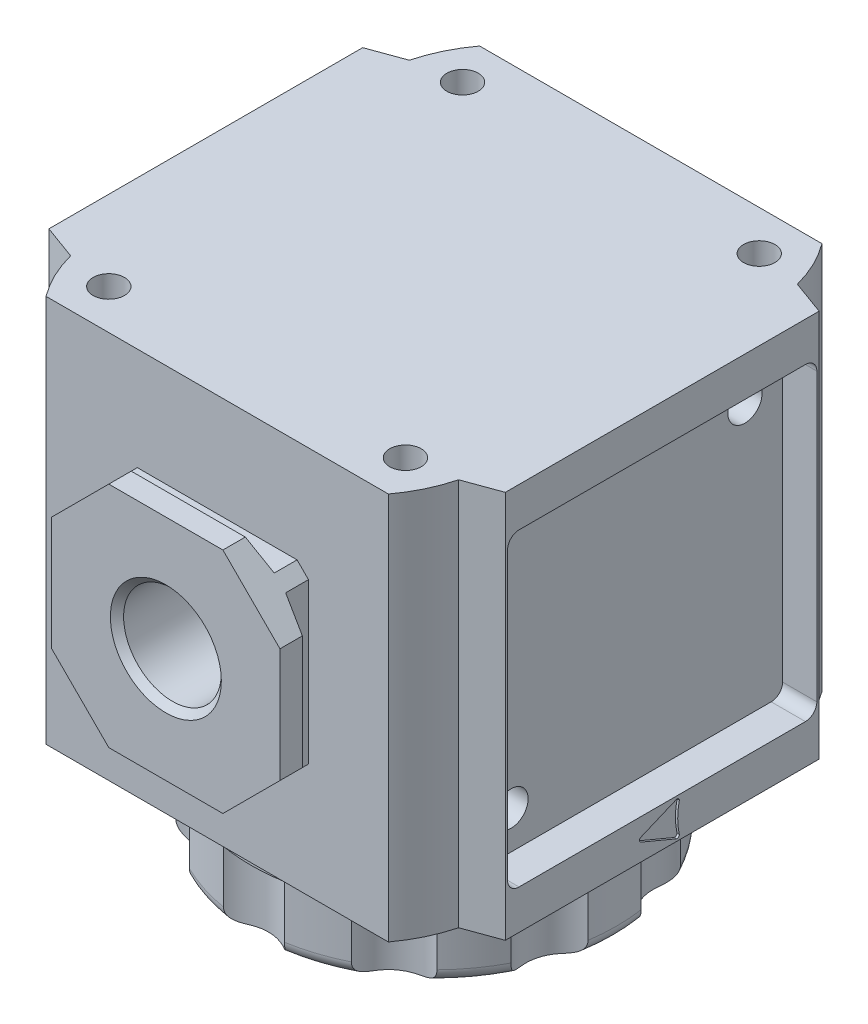
from build123d import *

# Parameters (mm, degrees)
EXTRUDE_1_DEPTH             = 17
EXTRUDE_1_DEPTH_BACK        = 17
EXTRUDE_2_DEPTH             = 17
EXTRUDE_2_DEPTH_BACK        = 17
EXTRUDE_3_DEPTH             = 17
EXTRUDE_3_DEPTH_BACK        = 17
SKETCH_5_R                  = 21.1
CUT_EXTRUDE_1_DEPTH         = 5.8
EXTRUDE_4_DEPTH             = 2
EXTRUDE_5_DEPTH             = 2.5
EXTRUDE_6_DEPTH             = 2
EXTRUDE_7_DEPTH             = 2.5
CUT_EXTRUDE_2_DEPTH         = 10
CUT_EXTRUDE_2_DEPTH_BACK    = 10
CUT_EXTRUDE_3_DEPTH         = 10
CUT_EXTRUDE_3_DEPTH_BACK    = 10
CUT_EXTRUDE_4_DEPTH         = 10
CUT_EXTRUDE_4_DEPTH_BACK    = 10
CUT_EXTRUDE_5_DEPTH         = 10
CUT_EXTRUDE_5_DEPTH_BACK    = 10
CUT_EXTRUDE_6_DEPTH         = 10
CUT_EXTRUDE_6_DEPTH_BACK    = 10
CUT_EXTRUDE_7_DEPTH         = 10
CUT_EXTRUDE_7_DEPTH_BACK    = 10
CUT_EXTRUDE_8_DEPTH         = 10
CUT_EXTRUDE_8_DEPTH_BACK    = 10
CUT_EXTRUDE_9_DEPTH         = 10
CUT_EXTRUDE_9_DEPTH_BACK    = 10
SKETCH_20_R                 = 1.5
CUT_EXTRUDE_10_DEPTH        = 6
SKETCH_21_R                 = 1.5
CUT_EXTRUDE_11_DEPTH        = 6
SKETCH_22_R                 = 1.375
CUT_EXTRUDE_12_DEPTH        = 3
PATTERN_LINEAR_1_COUNT      = 2
PATTERN_LINEAR_1_PITCH      = 26
PATTERN_LINEAR_1_COUNT_DIR2 = 2
PATTERN_LINEAR_1_PITCH_DIR2 = 31
SKETCH_24_R                 = 13
CUT_EXTRUDE_13_DEPTH        = 0.2
CUT_EXTRUDE_14_DEPTH        = 0.2
CUT_EXTRUDE_15_DEPTH        = 0.2
CUT_EXTRUDE_16_DEPTH        = 1
EXTRUDE_8_DEPTH             = 1
SKETCH_29_R                 = 1.5
CUT_EXTRUDE_17_DEPTH        = 0.5
SKETCH_31_R                 = 1.5
CUT_EXTRUDE_18_DEPTH        = 0.5
SKETCH_30_R                 = 0.271317829
CUT_EXTRUDE_19_DEPTH        = 0.2
CUT_EXTRUDE_20_DEPTH        = 3


with BuildPart() as part:
    # 草图1 → 凸台-拉伸1 (new, two sides: drawn at the far end of the back side and taken through both)
    with BuildSketch(Plane(origin=(0, 0, 0), x_dir=(1, 0, 0), z_dir=(0, 1, 0)).offset(-EXTRUDE_1_DEPTH_BACK)):
        with BuildLine():
            Line((-17, 14.841910703), (-17, -14.841910703))
            ThreePointArc((-17, -14.841910703), (-16.201733132, -17.017987001), (-15, -19))
            Line((-15, -19), (15, -19))
            ThreePointArc((15, -19), (16.201733132, -17.017987001), (17, -14.841910703))
            Line((17, -14.841910703), (17, 14.841910703))
            ThreePointArc((17, 14.841910703), (16.201733132, 17.017987001), (15, 19))
            Line((15, 19), (-15, 19))
            ThreePointArc((-15, 19), (-16.201733132, 17.017987001), (-17, 14.841910703))
        make_face()
    extrude(amount=EXTRUDE_1_DEPTH + EXTRUDE_1_DEPTH_BACK)

    # 草图2 → 凸台-拉伸2 (add, two sides: drawn at the far end of the back side and taken through both)
    with BuildSketch(Plane(origin=(0, 0, 0), x_dir=(1, 0, 0), z_dir=(0, 1, 0)).offset(-EXTRUDE_2_DEPTH_BACK)):
        Polygon((-20, -13.75), (-17, -14.841910703), (-17, 14.841910703), (-20, 13.75), align=None)
    extrude(amount=EXTRUDE_2_DEPTH + EXTRUDE_2_DEPTH_BACK)

    # 草图3 → 凸台-拉伸3 (add, two sides: drawn at the far end of the back side and taken through both)
    with BuildSketch(Plane(origin=(0, 0, 0), x_dir=(1, 0, 0), z_dir=(0, 1, 0)).offset(-EXTRUDE_3_DEPTH_BACK)):
        Polygon((17, 14.841910703), (17, -14.841910703), (20, -13.75), (20, 13.75), align=None)
    extrude(amount=EXTRUDE_3_DEPTH + EXTRUDE_3_DEPTH_BACK)

    # 草图4 → 旋转1 (revolve)
    with BuildSketch(Plane.XY, mode=Mode.PRIVATE) as revolve_1_sk:
        with BuildLine():
            Line((0, -17), (16.1, -17))
            Line((16.1, -17), (16.1, -19))
            Line((16.1, -19), (16, -19))
            Line((16, -19), (16, -24.8))
            ThreePointArc((16, -24.8), (15.648528137, -25.648528137), (14.8, -26))
            Line((14.8, -26), (0, -26))
            Line((0, -26), (0, -17))
        make_face()
    revolve(revolve_1_sk.sketch.rotate(Axis((0, -26, 0), (0, 1, 0)), 270), axis=Axis((0, -26, 0), (0, 1, 0)))

    # 草图5 → 切除-拉伸1 (cut)
    with BuildSketch(Plane(origin=(0, -26, 0), x_dir=(-1, 0, 0), z_dir=(0, -1, 0))):
        Circle(SKETCH_5_R)
        with BuildLine():
            ThreePointArc((15.830577633, -2.322242841), (16, 0), (15.830577633, 2.322242841))
            ThreePointArc((15.830577633, 2.322242841), (13.790319486, 4.480746418), (14.17218643, 7.426246145))
            ThreePointArc((14.17218643, 7.426246145), (12.94427191, 9.404564037), (11.442226242, 11.183713991))
            ThreePointArc((11.442226242, 11.183713991), (8.522886158, 11.730746418), (7.100501705, 14.338161512))
            ThreePointArc((7.100501705, 14.338161512), (4.94427191, 15.216904261), (2.683333333, 15.773386517))
            ThreePointArc((2.683333333, 15.773386517), (0, 14.5), (-2.683333333, 15.773386517))
            ThreePointArc((-2.683333333, 15.773386517), (-4.94427191, 15.216904261), (-7.100501705, 14.338161512))
            ThreePointArc((-7.100501705, 14.338161512), (-8.522886158, 11.730746418), (-11.442226242, 11.183713991))
            ThreePointArc((-11.442226242, 11.183713991), (-12.94427191, 9.404564037), (-14.17218643, 7.426246145))
            ThreePointArc((-14.17218643, 7.426246145), (-13.790319486, 4.480746418), (-15.830577633, 2.322242841))
            ThreePointArc((-15.830577633, 2.322242841), (-16, 0), (-15.830577633, -2.322242841))
            ThreePointArc((-15.830577633, -2.322242841), (-13.790319486, -4.480746418), (-14.17218643, -7.426246145))
            ThreePointArc((-14.17218643, -7.426246145), (-12.94427191, -9.404564037), (-11.442226242, -11.183713991))
            ThreePointArc((-11.442226242, -11.183713991), (-8.522886158, -11.730746418), (-7.100501705, -14.338161512))
            ThreePointArc((-7.100501705, -14.338161512), (-4.94427191, -15.216904261), (-2.683333333, -15.773386517))
            ThreePointArc((-2.683333333, -15.773386517), (0, -14.5), (2.683333333, -15.773386517))
            ThreePointArc((2.683333333, -15.773386517), (4.94427191, -15.216904261), (7.100501705, -14.338161512))
            ThreePointArc((7.100501705, -14.338161512), (8.522886158, -11.730746418), (11.442226242, -11.183713991))
            ThreePointArc((11.442226242, -11.183713991), (12.94427191, -9.404564037), (14.17218643, -7.426246145))
            ThreePointArc((14.17218643, -7.426246145), (13.790319486, -4.480746418), (15.830577633, -2.322242841))
        make_face(mode=Mode.SUBTRACT)
    extrude(amount=-CUT_EXTRUDE_1_DEPTH, mode=Mode.SUBTRACT)

    # 草图6 → 凸台-拉伸4 (add)
    with BuildSketch(Plane.XY.offset(19)):
        Polygon((-8, -7), (-7, -8), (7, -8), (8, -7), (8, 7), (7, 8), (-7, 8), (-8, 7), align=None)
    extrude(amount=EXTRUDE_4_DEPTH)

    # 草图7 → 凸台-拉伸5 (add)
    with BuildSketch(Plane.XY.offset(21)):
        Polygon((-10, -5), (-5, -10), (5, -10), (10, -5), (10, 5), (5, 10), (-5, 10), (-10, 5), align=None)
    extrude(amount=EXTRUDE_5_DEPTH)

    # 草图8 → 凸台-拉伸6 (add)
    with BuildSketch(Plane.XY.offset(-19)):
        Polygon((-8, -7), (-7, -8), (7, -8), (8, -7), (8, 7), (7, 8), (-7, 8), (-8, 7), align=None)
    extrude(amount=-EXTRUDE_6_DEPTH)

    # 草图9 → 凸台-拉伸7 (add)
    with BuildSketch(Plane.XY.offset(-21)):
        Polygon((-10, -5), (-5, -10), (5, -10), (10, -5), (10, 5), (5, 10), (-5, 10), (-10, 5), align=None)
    extrude(amount=-EXTRUDE_7_DEPTH)

    # 草图10 → 切除-拉伸2 (cut, two sides: drawn at the far end of the back side and taken through both)
    with BuildSketch(Plane(origin=(0, 0, 0), x_dir=(0, 0, -1), z_dir=(1, 0, 0)).offset(-CUT_EXTRUDE_2_DEPTH_BACK)):
        Polygon((-21.535898385, 10), (-21, 8), (-21, 10), align=None)
    extrude(amount=CUT_EXTRUDE_2_DEPTH + CUT_EXTRUDE_2_DEPTH_BACK, mode=Mode.SUBTRACT)

    # 草图11 → 切除-拉伸3 (cut, two sides: drawn at the far end of the back side and taken through both)
    with BuildSketch(Plane(origin=(0, 0, 0), x_dir=(0, 0, -1), z_dir=(1, 0, 0)).offset(-CUT_EXTRUDE_3_DEPTH_BACK)):
        Polygon((-21.535898385, -10), (-21, -10), (-21, -8), align=None)
    extrude(amount=CUT_EXTRUDE_3_DEPTH + CUT_EXTRUDE_3_DEPTH_BACK, mode=Mode.SUBTRACT)

    # 草图12 → 切除-拉伸4 (cut, two sides: drawn at the far end of the back side and taken through both)
    with BuildSketch(Plane(origin=(0, 0, 0), x_dir=(0, 0, -1), z_dir=(1, 0, 0)).offset(-CUT_EXTRUDE_4_DEPTH_BACK)):
        Polygon((21, 8), (21.535898385, 10), (21, 10), align=None)
    extrude(amount=CUT_EXTRUDE_4_DEPTH + CUT_EXTRUDE_4_DEPTH_BACK, mode=Mode.SUBTRACT)

    # 草图13 → 切除-拉伸5 (cut, two sides: drawn at the far end of the back side and taken through both)
    with BuildSketch(Plane(origin=(0, 0, 0), x_dir=(0, 0, -1), z_dir=(1, 0, 0)).offset(-CUT_EXTRUDE_5_DEPTH_BACK)):
        Polygon((21, -8), (21, -10), (21.535898385, -10), align=None)
    extrude(amount=CUT_EXTRUDE_5_DEPTH + CUT_EXTRUDE_5_DEPTH_BACK, mode=Mode.SUBTRACT)

    # 草图14 → 切除-拉伸6 (cut, two sides: drawn at the far end of the back side and taken through both)
    with BuildSketch(Plane(origin=(0, 0, 0), x_dir=(1, 0, 0), z_dir=(0, 1, 0)).offset(-CUT_EXTRUDE_6_DEPTH_BACK)):
        Polygon((8, 21), (10, 21), (10, 21.535898385), align=None)
    extrude(amount=CUT_EXTRUDE_6_DEPTH + CUT_EXTRUDE_6_DEPTH_BACK, mode=Mode.SUBTRACT)

    # 草图15 → 切除-拉伸7 (cut, two sides: drawn at the far end of the back side and taken through both)
    with BuildSketch(Plane(origin=(0, 0, 0), x_dir=(1, 0, 0), z_dir=(0, 1, 0)).offset(-CUT_EXTRUDE_7_DEPTH_BACK)):
        Polygon((-10, 21), (-8, 21), (-10, 21.535898385), align=None)
    extrude(amount=CUT_EXTRUDE_7_DEPTH + CUT_EXTRUDE_7_DEPTH_BACK, mode=Mode.SUBTRACT)

    # 草图16 → 切除-拉伸8 (cut, two sides: drawn at the far end of the back side and taken through both)
    with BuildSketch(Plane(origin=(0, 0, 0), x_dir=(1, 0, 0), z_dir=(0, 1, 0)).offset(-CUT_EXTRUDE_8_DEPTH_BACK)):
        Polygon((8, -21), (10, -21.535898385), (10, -21), align=None)
    extrude(amount=CUT_EXTRUDE_8_DEPTH + CUT_EXTRUDE_8_DEPTH_BACK, mode=Mode.SUBTRACT)

    # 草图17 → 切除-拉伸9 (cut, two sides: drawn at the far end of the back side and taken through both)
    with BuildSketch(Plane(origin=(0, 0, 0), x_dir=(1, 0, 0), z_dir=(0, 1, 0)).offset(-CUT_EXTRUDE_9_DEPTH_BACK)):
        Polygon((-10, -21), (-10, -21.535898385), (-8, -21), align=None)
    extrude(amount=CUT_EXTRUDE_9_DEPTH + CUT_EXTRUDE_9_DEPTH_BACK, mode=Mode.SUBTRACT)

    # 草图18 → 切除-旋转1 (revolve, cut)
    with BuildSketch(Plane(origin=(0, 0, 0), x_dir=(0, 0, -1), z_dir=(1, 0, 0)), mode=Mode.PRIVATE) as cut_revolve_1_sk:
        Polygon((14.5, 0), (14.5, 4.283), (22.919, 4.283), (23.5, 4.864), (23.5, 0), align=None)
    revolve(cut_revolve_1_sk.sketch.rotate(Axis((0, 0, -23.5), (0, 0, 1)), 270), axis=Axis((0, 0, -23.5), (0, 0, 1)), mode=Mode.SUBTRACT)

    # 草图19 → 切除-旋转2 (revolve, cut)
    with BuildSketch(Plane(origin=(0, 0, 0), x_dir=(0, 0, -1), z_dir=(1, 0, 0)), mode=Mode.PRIVATE) as cut_revolve_2_sk:
        Polygon((-23.5, 0), (-23.5, 4.864), (-22.919, 4.283), (-14.5, 4.283), (-14.5, 0), align=None)
    revolve(cut_revolve_2_sk.sketch.rotate(Axis((0, 0, 14.5), (0, 0, 1)), 270), axis=Axis((0, 0, 14.5), (0, 0, 1)), mode=Mode.SUBTRACT)

    # 草图20 → 切除-拉伸10 (cut)
    with BuildSketch(Plane(origin=(20, 0, 0), x_dir=(0, 0, -1), z_dir=(1, 0, 0))):
        with Locations((10.25, 10.25)):
            Circle(SKETCH_20_R)
    extrude(amount=-CUT_EXTRUDE_10_DEPTH, mode=Mode.SUBTRACT)

    # 草图21 → 切除-拉伸11 (cut)
    with BuildSketch(Plane(origin=(20, 0, 0), x_dir=(0, 0, -1), z_dir=(1, 0, 0))):
        with Locations((-10.25, -10.25)):
            Circle(SKETCH_21_R)
    extrude(amount=-CUT_EXTRUDE_11_DEPTH, mode=Mode.SUBTRACT)

    # 草图22 → 切除-拉伸12 (cut)
    with BuildSketch(Plane(origin=(0, 17, 0), x_dir=(1, 0, 0), z_dir=(0, 1, 0))):
        with Locations(Location((13, 15.5, 0), (0, 0, 270))):
            Circle(SKETCH_22_R)
    cut_extrude_12 = extrude(amount=-CUT_EXTRUDE_12_DEPTH, mode=Mode.SUBTRACT)

    # 阵列(线性)1: Cut-Extrude 12 2 × 2
    with Locations(*[(-i * PATTERN_LINEAR_1_PITCH, 0, j * PATTERN_LINEAR_1_PITCH_DIR2) for i in range(PATTERN_LINEAR_1_COUNT) for j in range(PATTERN_LINEAR_1_COUNT_DIR2) if (i, j) != (0, 0)]):
        add(cut_extrude_12, mode=Mode.SUBTRACT)

    # 草图24 → 切除-拉伸13 (cut)
    with BuildSketch(Plane(origin=(0, -26, 0), x_dir=(1, 0, 0), z_dir=(0, 1, 0))):
        with Locations(Location((0, 0, 0), (0, 0, 270))):
            Circle(SKETCH_24_R)
        with BuildLine():
            Line((-6.231307442, -4.53908708), (-0.029757054, -4.53908708))
            Line((-0.029757054, -4.53908708), (1.051022371, -2.058466925))
            Line((1.051022371, -2.058466925), (-1.768230231, -2.058466925))
            Line((-1.768230231, -2.058466925), (0, 2))
            Line((0, 2), (2.798913614, -4.53908708))
            Line((2.798913614, -4.53908708), (6.171793333, -4.53908708))
            Line((6.171793333, -4.53908708), (1.437936027, 6.520598718))
            ThreePointArc((1.437936027, 6.520598718), (0.01763004, 7.460904841), (-1.408717665, 6.529788884))
            Line((-1.408717665, 6.529788884), (-6.231307442, -4.53908708))
        make_face(mode=Mode.SUBTRACT)
    extrude(amount=CUT_EXTRUDE_13_DEPTH, mode=Mode.SUBTRACT)

    # 草图25 → 切除-拉伸14 (cut)
    with BuildSketch(Plane(origin=(20, 0, 0), x_dir=(0, 0, -1), z_dir=(1, 0, 0))):
        with BuildLine():
            Line((-1.877345335, -15.484438876), (1.222654665, -16.784438876))
            ThreePointArc((1.222654665, -16.784438876), (1.410749566, -16.766536883), (1.5, -16.6))
            ThreePointArc((1.5, -16.6), (1.357473858, -15.3), (1.5, -14))
            ThreePointArc((1.5, -14), (1.410749566, -13.833463117), (1.222654665, -13.815561124))
            Line((1.222654665, -13.815561124), (-1.877345335, -15.115561124))
            ThreePointArc((-1.877345335, -15.115561124), (-2, -15.3), (-1.877345335, -15.484438876))
        make_face()
    extrude(amount=-CUT_EXTRUDE_14_DEPTH, mode=Mode.SUBTRACT)

    # 草图26 → 切除-拉伸15 (cut)
    with BuildSketch(Plane(origin=(-20, 0, 0), x_dir=(0, 0, -1), z_dir=(1, 0, 0))):
        with BuildLine():
            Line((-1.222654665, -15.984438876), (1.877345335, -14.684438876))
            ThreePointArc((1.877345335, -14.684438876), (2, -14.5), (1.877345335, -14.315561124))
            Line((1.877345335, -14.315561124), (-1.222654665, -13.015561124))
            ThreePointArc((-1.222654665, -13.015561124), (-1.410749566, -13.033463117), (-1.5, -13.2))
            ThreePointArc((-1.5, -13.2), (-1.357473858, -14.5), (-1.5, -15.8))
            ThreePointArc((-1.5, -15.8), (-1.410749566, -15.966536883), (-1.222654665, -15.984438876))
        make_face()
    extrude(amount=CUT_EXTRUDE_15_DEPTH, mode=Mode.SUBTRACT)

    # 草图27 → 切除-拉伸16 (cut)
    with BuildSketch(Plane(origin=(-20, 0, 0), x_dir=(0, 0, -1), z_dir=(1, 0, 0))):
        with BuildLine():
            Line((-12.5, 11.5), (-12.5, -11.5))
            ThreePointArc((-12.5, -11.5), (-12.207106781, -12.207106781), (-11.5, -12.5))
            Line((-11.5, -12.5), (11.5, -12.5))
            ThreePointArc((11.5, -12.5), (12.207106781, -12.207106781), (12.5, -11.5))
            Line((12.5, -11.5), (12.5, 11.5))
            ThreePointArc((12.5, 11.5), (12.207106781, 12.207106781), (11.5, 12.5))
            Line((11.5, 12.5), (-11.5, 12.5))
            ThreePointArc((-11.5, 12.5), (-12.207106781, 12.207106781), (-12.5, 11.5))
        make_face()
    extrude(amount=CUT_EXTRUDE_16_DEPTH, mode=Mode.SUBTRACT)

    # 草图28 → 凸台-拉伸8 (add)
    with BuildSketch(Plane(origin=(-20, 0, 0), x_dir=(0, 0, -1), z_dir=(1, 0, 0))):
        with BuildLine():
            Line((-12.25, 11.27), (-12.25, -11.27))
            ThreePointArc((-12.25, -11.27), (-11.962964646, -11.962964646), (-11.27, -12.25))
            Line((-11.27, -12.25), (11.27, -12.25))
            ThreePointArc((11.27, -12.25), (11.962964646, -11.962964646), (12.25, -11.27))
            Line((12.25, -11.27), (12.25, 11.27))
            ThreePointArc((12.25, 11.27), (11.962964646, 11.962964646), (11.27, 12.25))
            Line((11.27, 12.25), (-11.27, 12.25))
            ThreePointArc((-11.27, 12.25), (-11.962964646, 11.962964646), (-12.25, 11.27))
        make_face()
    extrude(amount=EXTRUDE_8_DEPTH)

    # 草图29 → 切除-拉伸17 (cut)
    with BuildSketch(Plane(origin=(-20, 0, 0), x_dir=(0, 0, -1), z_dir=(1, 0, 0))):
        with Locations((-10.25, 10.25)):
            Circle(SKETCH_29_R)
        with BuildLine():
            Line((-8.914897008, 10.05), (-11.585102992, 10.05))
            ThreePointArc((-11.585102992, 10.05), (-10.25, 8.9), (-8.914897008, 10.05))
        make_face(mode=Mode.SUBTRACT)
        with BuildLine():
            Line((-11.585102992, 10.45), (-8.914897008, 10.45))
            ThreePointArc((-8.914897008, 10.45), (-10.25, 11.6), (-11.585102992, 10.45))
        make_face(mode=Mode.SUBTRACT)
    extrude(amount=CUT_EXTRUDE_17_DEPTH, mode=Mode.SUBTRACT)

    # 草图31 → 切除-拉伸18 (cut)
    with BuildSketch(Plane(origin=(-20, 0, 0), x_dir=(0, 0, -1), z_dir=(1, 0, 0))):
        with Locations((10.25, -10.25)):
            Circle(SKETCH_31_R)
        with BuildLine():
            Line((8.914897008, -10.05), (11.585102992, -10.05))
            ThreePointArc((11.585102992, -10.05), (10.25, -8.9), (8.914897008, -10.05))
        make_face(mode=Mode.SUBTRACT)
        with BuildLine():
            Line((11.585102992, -10.45), (8.914897008, -10.45))
            ThreePointArc((8.914897008, -10.45), (10.25, -11.6), (11.585102992, -10.45))
        make_face(mode=Mode.SUBTRACT)
    extrude(amount=CUT_EXTRUDE_18_DEPTH, mode=Mode.SUBTRACT)

    # 草图30 → 切除-拉伸19 (cut)
    with BuildSketch(Plane(origin=(-20, 0, 0), x_dir=(0, 0, -1), z_dir=(1, 0, 0))):
        with BuildLine():
            ThreePointArc((-5.905423792, 1.004597585), (-6.3, 0), (-5.905423792, -1.004597585))
            ThreePointArc((-5.905423792, -1.004597585), (0, -2.8), (5.905423792, -1.004597585))
            ThreePointArc((5.905423792, -1.004597585), (6.3, 0), (5.905423792, 1.004597585))
            ThreePointArc((5.905423792, 1.004597585), (0, 2.8), (-5.905423792, 1.004597585))
        make_face()
        with Locations((-2.330321537, -0.933333333)):
            Circle(SKETCH_30_R, mode=Mode.SUBTRACT)
        with BuildLine():
            Line((3.340221098, -1.204651163), (4.262701719, -1.204651163))
            ThreePointArc((4.262701719, -1.204651163), (4.377812125, -1.156970871), (4.425492416, -1.041860465))
            Line((4.425492416, -1.041860465), (4.425492416, -0.526356589))
            ThreePointArc((4.425492416, -0.526356589), (4.361918694, -0.372876047), (4.208438153, -0.309302326))
            Line((4.208438153, -0.309302326), (4.19758544, -0.309302326))
            ThreePointArc((4.19758544, -0.309302326), (4.044104898, -0.372876047), (3.980531176, -0.526356589))
            Line((3.980531176, -0.526356589), (3.980531176, -0.733510478))
            Line((3.980531176, -0.733510478), (3.627817998, -0.733510478))
            Line((3.627817998, -0.733510478), (3.627817998, 0.406024406))
            Line((3.627817998, 0.406024406), (3.980531176, 0.406024406))
            Line((3.980531176, 0.406024406), (3.980531176, 0.217054264))
            ThreePointArc((3.980531176, 0.217054264), (4.044104898, 0.063573722), (4.19758544, 0))
            Line((4.19758544, 0), (4.208438153, 0))
            ThreePointArc((4.208438153, 0), (4.361918694, 0.063573722), (4.425492416, 0.217054264))
            Line((4.425492416, 0.217054264), (4.425492416, 0.73255814))
            ThreePointArc((4.425492416, 0.73255814), (4.377812125, 0.847668546), (4.262701719, 0.895348837))
            Line((4.262701719, 0.895348837), (3.340221098, 0.895348837))
            ThreePointArc((3.340221098, 0.895348837), (3.225110692, 0.847668546), (3.177430401, 0.73255814))
            Line((3.177430401, 0.73255814), (3.177430401, -1.041860465))
            ThreePointArc((3.177430401, -1.041860465), (3.225110692, -1.156970871), (3.340221098, -1.204651163))
        make_face(mode=Mode.SUBTRACT)
        with BuildLine():
            Line((0.898360633, 0.895348837), (1.742313844, -1.041704456))
            ThreePointArc((1.742313844, -1.041704456), (1.991924693, -1.204649749), (2.24047824, -1.040096177))
            Line((2.24047824, -1.040096177), (3.068903269, 0.895348837))
            Line((3.068903269, 0.895348837), (2.478649318, 0.895348837))
            Line((2.478649318, 0.895348837), (1.988839436, -0.248991402))
            Line((1.988839436, -0.248991402), (1.679399145, 0.46124031))
            Line((1.679399145, 0.46124031), (2.172768351, 0.46124031))
            Line((2.172768351, 0.46124031), (1.983631951, 0.895348837))
            Line((1.983631951, 0.895348837), (0.898360633, 0.895348837))
        make_face(mode=Mode.SUBTRACT)
        with BuildLine():
            Line((-0.51249208, -0.90620155), (-0.51249208, -0.960465116))
            ThreePointArc((-0.51249208, -0.960465116), (-0.440971643, -1.133130726), (-0.268306033, -1.204651163))
            Line((-0.268306033, -1.204651163), (0.925492416, -1.204651163))
            ThreePointArc((0.925492416, -1.204651163), (1.098158026, -1.133130726), (1.169678463, -0.960465116))
            Line((1.169678463, -0.960465116), (1.169678463, -0.90620155))
            ThreePointArc((1.169678463, -0.90620155), (1.098158026, -0.733535941), (0.925492416, -0.662015504))
            Line((0.925492416, -0.662015504), (0.599911021, -0.662015504))
            Line((0.599911021, -0.662015504), (0.599911021, 0.895348837))
            Line((0.599911021, 0.895348837), (0.057275362, 0.895348837))
            Line((0.057275362, 0.895348837), (0.057275362, -0.662015504))
            Line((0.057275362, -0.662015504), (-0.268306033, -0.662015504))
            ThreePointArc((-0.268306033, -0.662015504), (-0.440971643, -0.733535941), (-0.51249208, -0.90620155))
        make_face(mode=Mode.SUBTRACT)
        with BuildLine():
            Line((-0.70241456, -1.204651163), (-0.70241456, -0.770542636))
            ThreePointArc((-0.70241456, -0.770542636), (-1.201226321, -0.563928039), (-1.407840917, -0.065116279))
            Line((-1.407840917, -0.065116279), (-1.407840917, 0.895348837))
            Line((-1.407840917, 0.895348837), (-1.787685878, 0.895348837))
            Line((-1.787685878, 0.895348837), (-1.787685878, -0.933333333))
            ThreePointArc((-1.787685878, -0.933333333), (-1.60009561, -1.19140902), (-1.296726178, -1.092615514))
            ThreePointArc((-1.296726178, -1.092615514), (-1.265279576, -1.071663027), (-1.227780007, -1.076318978))
            ThreePointArc((-1.227780007, -1.076318978), (-0.972820738, -1.172103294), (-0.70241456, -1.204651163))
        make_face(mode=Mode.SUBTRACT)
        with BuildLine():
            Line((-2.35745332, -0.569767442), (-2.303189754, -0.569767442))
            ThreePointArc((-2.303189754, -0.569767442), (-2.130524145, -0.498247005), (-2.059003708, -0.325581395))
            Line((-2.059003708, -0.325581395), (-2.059003708, 0.895348837))
            Line((-2.059003708, 0.895348837), (-2.601639367, 0.895348837))
            Line((-2.601639367, 0.895348837), (-2.601639367, -0.325581395))
            ThreePointArc((-2.601639367, -0.325581395), (-2.53011893, -0.498247005), (-2.35745332, -0.569767442))
        make_face(mode=Mode.SUBTRACT)
        with BuildLine():
            Line((-4.962104483, 0.895348837), (-4.118151272, -1.041704456))
            ThreePointArc((-4.118151272, -1.041704456), (-3.868540424, -1.204649749), (-3.619986876, -1.040096177))
            Line((-3.619986876, -1.040096177), (-2.791561847, 0.895348837))
            Line((-2.791561847, 0.895348837), (-3.381815798, 0.895348837))
            Line((-3.381815798, 0.895348837), (-3.871625681, -0.248991402))
            Line((-3.871625681, -0.248991402), (-4.181065971, 0.46124031))
            Line((-4.181065971, 0.46124031), (-3.687696766, 0.46124031))
            Line((-3.687696766, 0.46124031), (-3.876833165, 0.895348837))
            Line((-3.876833165, 0.895348837), (-4.962104483, 0.895348837))
        make_face(mode=Mode.SUBTRACT)
    extrude(amount=CUT_EXTRUDE_19_DEPTH, mode=Mode.SUBTRACT)

    # 草图32 → 切除-拉伸20 (cut)
    with BuildSketch(Plane(origin=(20, 0, 0), x_dir=(0, 0, -1), z_dir=(1, 0, 0))):
        with BuildLine():
            Line((-13.55, 12.55), (-13.55, -12.55))
            ThreePointArc((-13.55, -12.55), (-13.257106781, -13.257106781), (-12.55, -13.55))
            Line((-12.55, -13.55), (12.55, -13.55))
            ThreePointArc((12.55, -13.55), (13.257106781, -13.257106781), (13.55, -12.55))
            Line((13.55, -12.55), (13.55, 12.55))
            ThreePointArc((13.55, 12.55), (13.257106781, 13.257106781), (12.55, 13.55))
            Line((12.55, 13.55), (-12.55, 13.55))
            ThreePointArc((-12.55, 13.55), (-13.257106781, 13.257106781), (-13.55, 12.55))
        make_face()
    extrude(amount=-CUT_EXTRUDE_20_DEPTH, mode=Mode.SUBTRACT)


solid = part.part
